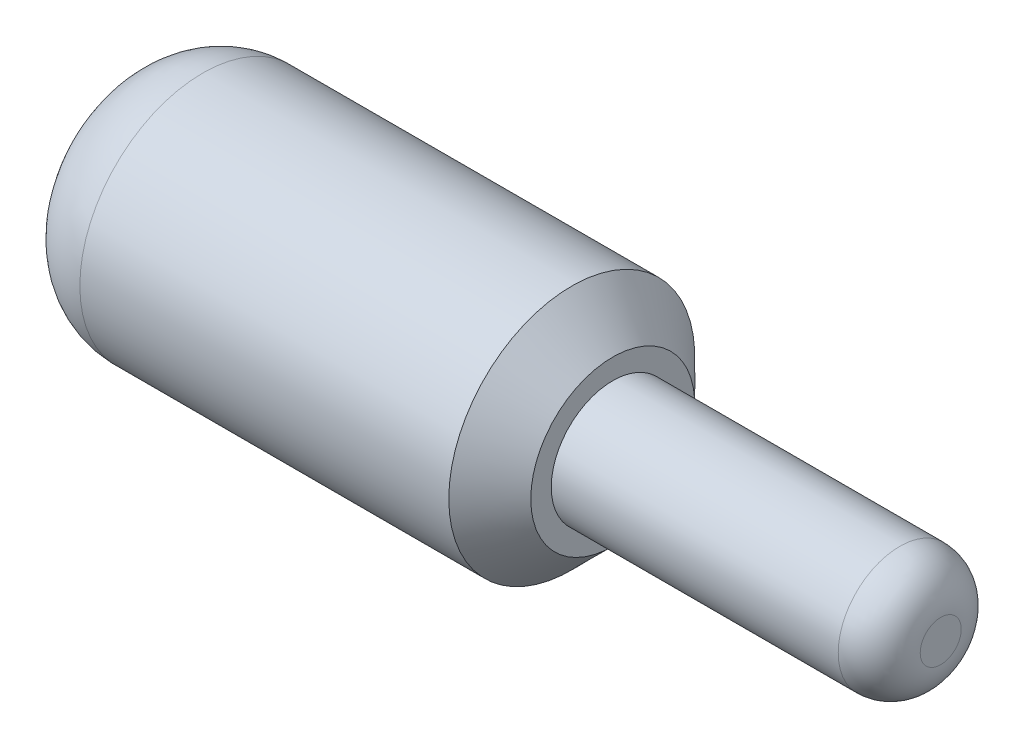
SolidWorks part; units mm, degrees
ref_plane "Front Plane" through (0, 0, 0) normal (0, 0, 1) x (1, 0, 0)
ref_plane "Top Plane" through (0, 0, 0) normal (0, 1, 0) x (1, 0, 0)
ref_plane "Right Plane" through (0, 0, 0) normal (1, 0, 0) x (0, 0, -1)
sketch "Sketch1" plane through (0, 0, 0) normal (0, 0, 1) x (1, 0, 0)
  line L0 (0, 0) -> (20, 0) construction
  line L1 (0, 0) -> (0, 3)
  line L2 (0, 3) -> (12, 3)
  line L3 (12, 3) -> (12, 1.5)
  line L4 (12, 1.5) -> (20, 1.5)
  line L5 (20, 1.5) -> (20, 0)
  line L6 (0, 0) -> (20, 0)
  dimension "D1" = 3
  dimension "D2" = 12
  dimension "D3" = 8
  dimension "D4" = 1.5
revolve "Revolve1" add sketch "Sketch1" angle 360 about L0
fillet "Fillet1" radius 2 1 edges at (0, 0, 3)
fillet "Fillet2" radius 1 1 edges at (20, 0, 1.5)
chamfer "Chamfer1" distance 1 angle 45 1 edges at (12, 0, 3)
